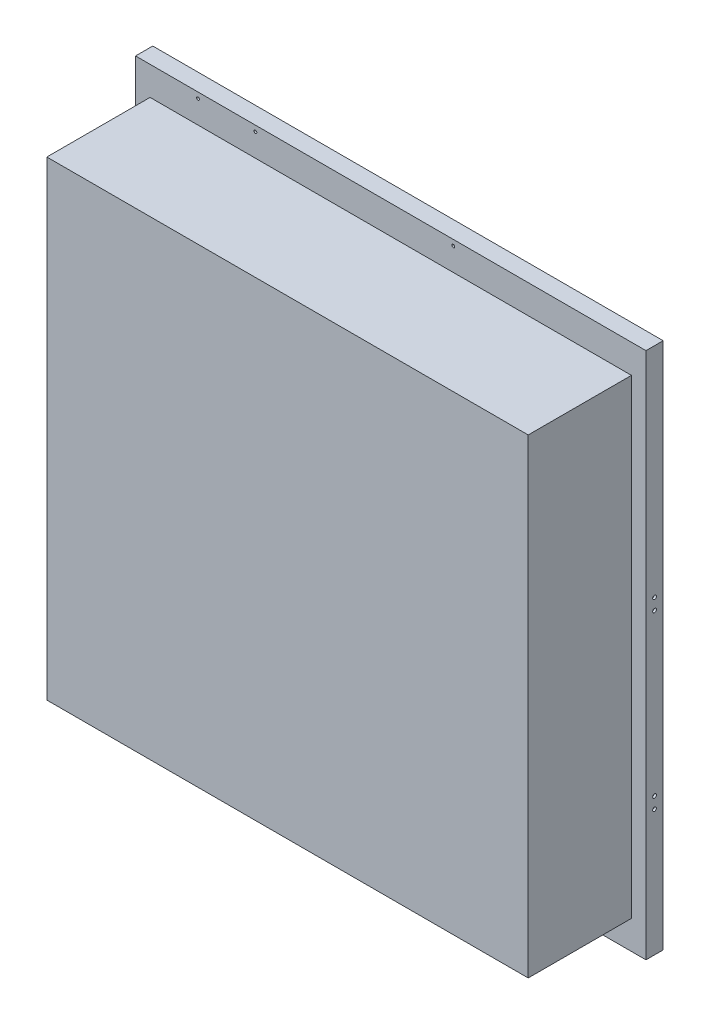
from build123d import *

# Parameters (mm, degrees)
SKETCH_1_W             = 445
SKETCH_1_H             = 470
EXTRUDE_1_DEPTH        = 7.5
SHELL_1_T              = 2
SKETCH_2_W             = 425
SKETCH_2_H             = 450
CUT_EXTRUDE_1_DEPTH    = 2
CUT_EXTRUDE_2_DEPTH    = 10
HOLE_WIZARD_M3_1_D     = 2.5
HOLE_WIZARD_M3_1_DEPTH = 7.5
SKETCH_9_W             = 445
SKETCH_9_H             = 5
CUT_EXTRUDE_4_DEPTH    = 324.969520171
SKETCH_10_W            = 445
SKETCH_10_H            = 15
EXTRUDE_2_DEPTH        = 1.5
SKETCH_11_W            = 445
SKETCH_11_H            = 15
EXTRUDE_3_DEPTH        = 1.5
MOVE_FACE_1_BY         = 5
MOVE_FACE_2_BY         = 5
EXTRUDE_4_DEPTH        = 2
HOLE_WIZARD_M4_1_D     = 3.3
HOLE_WIZARD_M3_2_D     = 2.5
HOLE_WIZARD_M3_3_D     = 2.5
PATTERN_LINEAR_1_COUNT = 2
PATTERN_LINEAR_1_PITCH = 10
HOLE_WIZARD_M3_4_D     = 2.5
SKETCH_26_W            = 419.683981368
SKETCH_26_H            = 410.034779602
EXTRUDE_5_DEPTH        = 90


with BuildPart() as part:
    # 草图1 → 凸台-拉伸1 (new, symmetric)
    with BuildSketch(Plane.XY):
        Rectangle(SKETCH_1_W, SKETCH_1_H)
    extrude(amount=EXTRUDE_1_DEPTH, both=True)

    # 抽壳1 (no face opened: a closed hollow body)
    add(offset(amount=-SHELL_1_T, mode=Mode.PRIVATE), mode=Mode.SUBTRACT)

    # 草图2 → 切除-拉伸1 (cut)
    with BuildSketch(Plane(origin=(0, 0, -7.5), x_dir=(-1, 0, 0), z_dir=(0, 0, -1))):
        Rectangle(SKETCH_2_W, SKETCH_2_H)
    extrude(amount=-CUT_EXTRUDE_1_DEPTH, mode=Mode.SUBTRACT)

    # 草图3 → 切除-拉伸2 (cut)
    with BuildSketch(Plane.XY.offset(7.5)):
        with BuildLine():
            Line((-205, 152.5), (-195, 152.5))
            ThreePointArc((-195, 152.5), (-192.5, 150), (-195, 147.5))
            Line((-195, 147.5), (-205, 147.5))
            ThreePointArc((-205, 147.5), (-207.5, 150), (-205, 152.5))
        make_face()
        with BuildLine():
            Line((195, 152.5), (205, 152.5))
            ThreePointArc((205, 152.5), (207.5, 150), (205, 147.5))
            Line((205, 147.5), (195, 147.5))
            ThreePointArc((195, 147.5), (192.5, 150), (195, 152.5))
        make_face()
        with BuildLine():
            Line((-205, -147.5), (-195, -147.5))
            ThreePointArc((-195, -147.5), (-192.5, -150), (-195, -152.5))
            Line((-195, -152.5), (-205, -152.5))
            ThreePointArc((-205, -152.5), (-207.5, -150), (-205, -147.5))
        make_face()
        with BuildLine():
            Line((195, -147.5), (205, -147.5))
            ThreePointArc((205, -147.5), (207.5, -150), (205, -152.5))
            Line((205, -152.5), (195, -152.5))
            ThreePointArc((195, -152.5), (192.5, -150), (195, -147.5))
        make_face()
    extrude(amount=-CUT_EXTRUDE_2_DEPTH, mode=Mode.SUBTRACT)

    # M3 螺纹孔1
    with Locations(Plane.XY.offset(7.5)):
        with Locations((-72.5, -215), (-172.5, -215), (37.5, -215), (147.5, -215), (193, -202.5), (147.5, -166.5), (66.5, -135), (-13.5, -135), (-58.5, -135), (-173.5, -135), (-182.5, -65), (-168, -15), (-118, -15), (-72.5, -65), (-81.5, -24), (37.5, -65), (15, -24), (49.5, -22.5), (147.5, -103.5), (193, -92.5), (147.5, -65), (162.5, -25), (193, 7.5), (193, 17.5), (193, 72.496566859), (162.5, 68), (152.5, 27), (134.5, 27), (100.5, 129), (49.5, 70.5), (193, 202.496566859), (152.5, 125), (134.5, 125), (54.5, 177), (54.5, 225), (4.5, 168.5), (-118, 225), (-168, 225)):
            Hole(HOLE_WIZARD_M3_1_D / 2, depth=HOLE_WIZARD_M3_1_DEPTH)

    # 草图9 → 切除-拉伸4 (cut, through all)
    with BuildSketch(Plane.XY.offset(7.5)):
        with Locations((0, 232.5)):
            Rectangle(SKETCH_9_W, SKETCH_9_H)
        with Locations((0, -232.5)):
            Rectangle(SKETCH_9_W, SKETCH_9_H)
    extrude(amount=-CUT_EXTRUDE_4_DEPTH, mode=Mode.SUBTRACT)

    # 草图10 → 凸台-拉伸2 (add)
    with BuildSketch(Plane(origin=(0, 230, 0), x_dir=(1, 0, 0), z_dir=(0, 1, 0))):
        Rectangle(SKETCH_10_W, SKETCH_10_H)
    extrude(amount=-EXTRUDE_2_DEPTH)

    # 草图11 → 凸台-拉伸3 (add)
    with BuildSketch(Plane.XZ.offset(230)):
        Rectangle(SKETCH_11_W, SKETCH_11_H)
    extrude(amount=-EXTRUDE_3_DEPTH)

    # Move Face 1: a face moved outward by 5.0
    extrude(part.faces().sort_by_distance((0, 225, -6.5))[0], amount=MOVE_FACE_1_BY, dir=(0, -1, 0))

    # Move Face 2: a face moved outward by 5.0
    extrude(part.faces().sort_by_distance((0, -225, -6.5))[0], amount=MOVE_FACE_2_BY, dir=(0, 1, 0))

    # 草图12 → 凸台-拉伸4 (add)
    with BuildSketch(Plane.XY.offset(7.5)):
        with BuildLine():
            Line((-195, 152.5), (-205, 152.5))
            ThreePointArc((-205, 152.5), (-207.5, 150), (-205, 147.5))
            Line((-205, 147.5), (-195, 147.5))
            ThreePointArc((-195, 147.5), (-192.5, 150), (-195, 152.5))
        make_face()
        with BuildLine():
            Line((-195, -147.5), (-205, -147.5))
            ThreePointArc((-205, -147.5), (-207.5, -150), (-205, -152.5))
            Line((-205, -152.5), (-195, -152.5))
            ThreePointArc((-195, -152.5), (-192.5, -150), (-195, -147.5))
        make_face()
        with BuildLine():
            Line((205, 152.5), (195, 152.5))
            ThreePointArc((195, 152.5), (192.5, 150), (195, 147.5))
            Line((195, 147.5), (205, 147.5))
            ThreePointArc((205, 147.5), (207.5, 150), (205, 152.5))
        make_face()
        with BuildLine():
            Line((205, -147.5), (195, -147.5))
            ThreePointArc((195, -147.5), (192.5, -150), (195, -152.5))
            Line((195, -152.5), (205, -152.5))
            ThreePointArc((205, -152.5), (207.5, -150), (205, -147.5))
        make_face()
    extrude(amount=-EXTRUDE_4_DEPTH)

    # M4 螺纹孔1 (through all)
    with Locations(Plane.ZY.offset(222.5)):
        with Locations((0, 30), (0, -120)):
            hole_wizard_m4_1 = Hole(HOLE_WIZARD_M4_1_D / 2)

    # M3 螺纹孔2 (through all)
    with Locations(Plane.XY.offset(7.5)):
        with Locations((-43.5, -135), (110, -135)):
            Hole(HOLE_WIZARD_M3_2_D / 2)

    # M3 螺纹孔3 (through all)
    with Locations(Plane.XY.offset(7.5)):
        with Locations((-71, 167.5)):
            Hole(HOLE_WIZARD_M3_3_D / 2)

    # 阵列(线性)1: M4 螺纹孔1 ×2
    with Locations(*[(0, i * PATTERN_LINEAR_1_PITCH, 0) for i in range(1, PATTERN_LINEAR_1_COUNT)]):
        add(hole_wizard_m4_1, mode=Mode.SUBTRACT)

    # M3 螺纹孔4 (through all)
    with Locations(Plane.XY.offset(7.5)):
        with Locations((109.5, 187), (137.5, 187), (109.5, -5), (137.5, -5)):
            Hole(HOLE_WIZARD_M3_4_D / 2)

    # 草图26 → 凸台-拉伸5 (add)
    with BuildSketch(Plane.XY.offset(7.5)):
        Rectangle(SKETCH_26_W, SKETCH_26_H)
    extrude(amount=EXTRUDE_5_DEPTH)


solid = part.part
